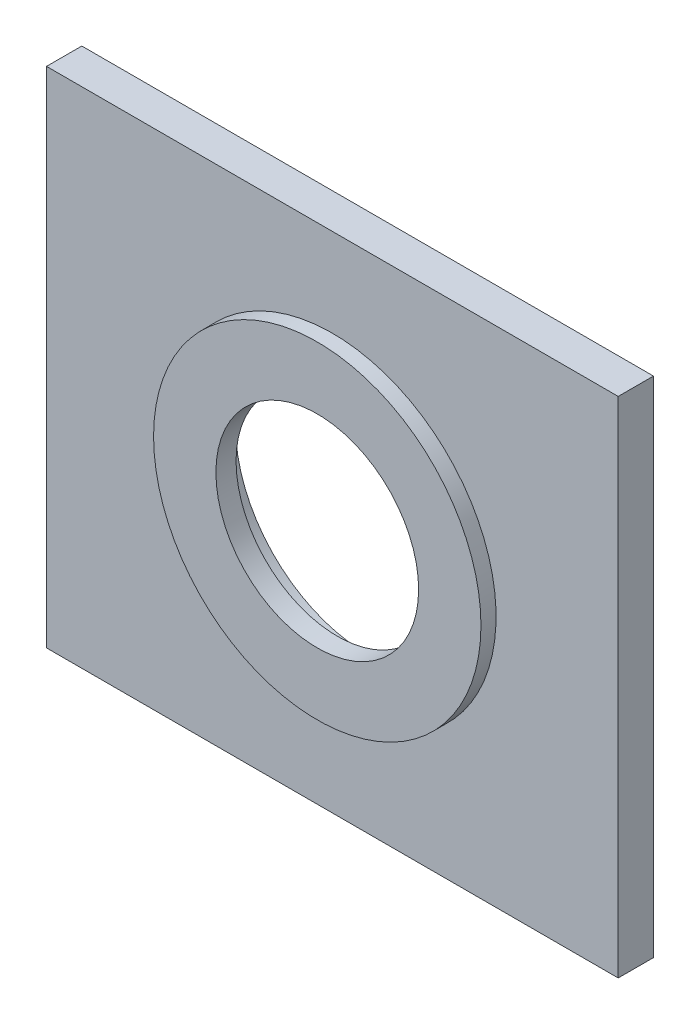
SolidWorks part; units mm, degrees
material "普通碳钢"
ref_plane "Front Plane" through (0, 0, 0) normal (0, 0, 1) x (1, 0, 0)
ref_plane "Top Plane" through (0, 0, 0) normal (0, 1, 0) x (1, 0, 0)
ref_plane "Right Plane" through (0, 0, 0) normal (1, 0, 0) x (0, 0, -1)
sketch "Sketch1" plane through (0, 0, 0) normal (0, 0, 1) x (1, 0, 0)
  line L0 (0, 0) -> (0, 200)
  line L1 (0, 200) -> (227, 200)
  line L2 (227, 200) -> (227, 0)
  line L3 (227, 0) -> (0, 0)
  dimension "D1" = 227
  dimension "D2" = 200
extrude "Boss-Extrude1" add sketch "Sketch1" along normal blind 14
sketch "Sketch2" plane through (0, 0, 14) normal (0, 0, 1) x (1, 0, 0)
  line L0 (0, 100) -> (227, 100) construction
  line L1 (0, 200) -> (0, 0) construction
  line L2 (227, 0) -> (227, 200) construction
  circle A0 centre (113.5, 100) radius 65
  dimension "D1" = 130
extrude "Boss-Extrude2" add sketch "Sketch2" along normal blind 6
sketch "Sketch3" plane through (0, 0, 0) normal (0, 0, -1) x (-1, 0, 0)
  circle A0 centre (-113.5, 100) radius 65 construction
  circle A1 centre (-113.5, 100) radius 65 construction
  circle A2 centre (-113.5, 100) radius 75
  circle A3 centre (-113.5, 100) radius 70
  dimension "D1" = 150
  dimension "D2" = 140
extrude "Boss-Extrude3" add sketch "Sketch3" along normal blind 8
sketch "Sketch4" plane through (0, 0, 20) normal (0, 0, 1) x (1, 0, 0)
  circle A0 centre (113.5, 100) radius 75 construction
  circle A1 centre (113.5, 100) radius 75 construction
  circle A2 centre (113.5, 100) radius 40.25
  dimension "D1" = 80.5
extrude "Cut-Extrude1" cut sketch "Sketch4" against normal through all
sketch "Sketch5" plane through (0, 0, 0) normal (0, 0, -1) x (-1, 0, 0)
  circle A0 centre (-113.5, 100) radius 52.5
  dimension "D1" = 105
extrude "Cut-Extrude2" cut sketch "Sketch5" against normal blind 12
